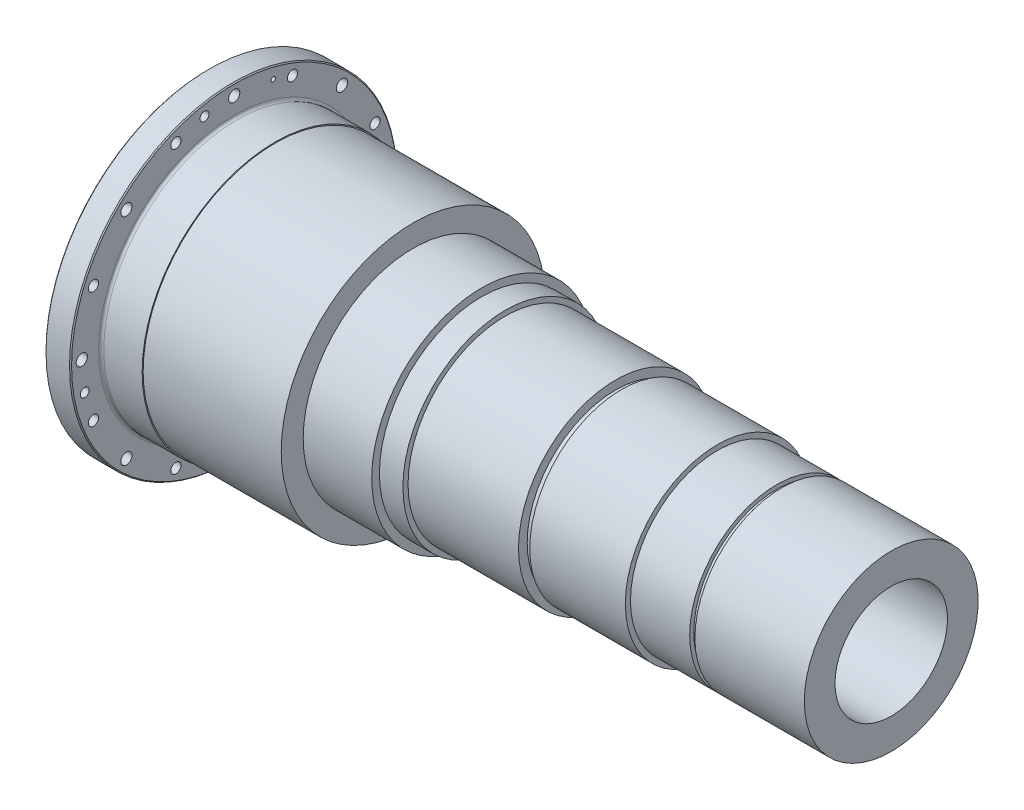
from build123d import *

# Parameters (mm, degrees)
M12_TAPPED_HOLE1_D     = 10.2
M12_TAPPED_HOLE1_DEPTH = 22
M12_TAPPED_HOLE1_TIP   = 3.064389157
M20_TAPPED_HOLE1_D     = 17.5
SKETCH3_R              = 10
SKETCH3_R_2            = 11
SKETCH3_R_3            = 4.25
CUT_EXTRUDE2_DEPTH     = 1410.618742781
SKETCH7_R              = 11.05
CUT_EXTRUDE3_DEPTH     = 2.75


with BuildPart() as part:
    # Sketch1 → Revolve1 (revolve)
    with BuildSketch(Plane.XY, mode=Mode.PRIVATE) as revolve1_sk:
        with BuildLine():
            Line((0, 203), (0, 318))
            Line((0, 318), (2, 320))
            Line((2, 320), (48, 320))
            Line((48, 320), (50, 318))
            Line((50, 318), (50, 265))
            ThreePointArc((50, 265), (51.464466094, 261.464466094), (55, 260))
            Line((55, 260), (130, 260))
            Line((130, 260), (130, 258))
            Line((130, 258), (400, 258))
            Line((400, 258), (400, 215))
            Line((400, 215), (534, 215))
            Line((534, 215), (534, 200))
            Line((534, 200), (580, 200))
            Line((580, 200), (580, 190))
            Line((580, 190), (796, 190))
            Line((796, 190), (796, 173))
            Line((796, 173), (808, 173))
            Line((808, 173), (808, 180))
            Line((808, 180), (995, 180))
            Line((995, 180), (995, 170))
            Line((995, 170), (1110.8, 170))
            Line((1110.8, 170), (1110.8, 162))
            Line((1110.8, 162), (1121, 162))
            Line((1121, 162), (1121, 170))
            Line((1121, 170), (1335, 170))
            Line((1335, 170), (1335, 110))
            Line((1335, 110), (874, 110))
            Line((874, 110), (864, 120))
            Line((864, 120), (413, 120))
            Line((413, 120), (413, 107.5))
            Line((413, 107.5), (353, 107.5))
            Line((353, 107.5), (353, 159))
            Line((353, 159), (340, 159))
            Line((340, 159), (340, 185))
            Line((340, 185), (283, 185))
            Line((283, 185), (283, 200))
            ThreePointArc((283, 200), (281.535533906, 203.535533906), (278, 205))
            Line((278, 205), (175, 205))
            ThreePointArc((175, 205), (171.464466094, 203.535533906), (170, 200))
            Line((170, 200), (170, 190))
            Line((170, 190), (110, 190))
            Line((110, 190), (110, 197))
            ThreePointArc((110, 197), (109.121320344, 199.121320344), (107, 200))
            Line((107, 200), (3, 200))
            Line((3, 200), (0, 203))
        make_face()
    revolve(revolve1_sk.sketch.rotate(Axis((0, 0, 0), (1, 0, 0)), 90), axis=Axis((0, 0, 0), (1, 0, 0)))

    # M12 Tapped Hole1
    with Locations(Plane(origin=(0, 58.136915961, 292.27401356), x_dir=(0, 0, -1), z_dir=(-1, 0, 0))):
        with Locations((0, 0)):
            Hole(M12_TAPPED_HOLE1_D / 2, depth=M12_TAPPED_HOLE1_DEPTH)
            with Locations((0, 0, -(M12_TAPPED_HOLE1_DEPTH + M12_TAPPED_HOLE1_TIP / 2))):  # 118° drill point
                Cone(0, M12_TAPPED_HOLE1_D / 2, M12_TAPPED_HOLE1_TIP, mode=Mode.SUBTRACT)

    # M20 Tapped Hole1 (through all)
    with Locations(Plane(origin=(0, 292.27401356, 58.136915961), x_dir=(0, 0, -1), z_dir=(-1, 0, 0))):
        with Locations((0, 0), (350.410929521, 234.137097599), (116.273831922, 584.54802712), (-234.137097599, 350.410929521)):
            Hole(M20_TAPPED_HOLE1_D / 2)

    # Sketch3 → Cut-Extrude2 (cut, through all)
    with BuildSketch(Plane.ZY):
        with Locations((114.039662845, 275.316100688)):
            Circle(SKETCH3_R)
        with Locations((0, 298)):
            Circle(SKETCH3_R_2)
        with Locations((210.717820794, 210.717820794)):
            Circle(SKETCH3_R_2)
        with Locations((275.316100688, 114.039662845)):
            Circle(SKETCH3_R)
        with Locations((298, 0)):
            Circle(SKETCH3_R_2)
        with Locations((275.316100688, -114.039662845)):
            Circle(SKETCH3_R)
        with Locations((210.717820794, -210.717820794)):
            Circle(SKETCH3_R_2)
        with Locations((114.039662845, -275.316100688)):
            Circle(SKETCH3_R)
        with Locations((0, -298)):
            Circle(SKETCH3_R_2)
        with Locations((-114.039662845, -275.316100688)):
            Circle(SKETCH3_R)
        with Locations((-210.717820794, -210.717820794)):
            Circle(SKETCH3_R_2)
        with Locations((-275.316100688, -114.039662845)):
            Circle(SKETCH3_R)
        with Locations((-298, 0)):
            Circle(SKETCH3_R_2)
        with Locations((-275.316100688, 114.039662845)):
            Circle(SKETCH3_R)
        with Locations((-210.717820794, 210.717820794)):
            Circle(SKETCH3_R_2)
        with Locations((-114.039662845, 275.316100688)):
            Circle(SKETCH3_R)
        with Locations((-76.5, 288.013454547)):
            Circle(SKETCH3_R_3)
    extrude(amount=-CUT_EXTRUDE2_DEPTH, mode=Mode.SUBTRACT)

    # Sketch7 → Cut-Extrude3 (cut)
    with BuildSketch(Plane.ZY):
        with Locations((-76.5, 288.013454547)):
            Circle(SKETCH7_R)
    extrude(amount=-CUT_EXTRUDE3_DEPTH, mode=Mode.SUBTRACT)


solid = part.part
